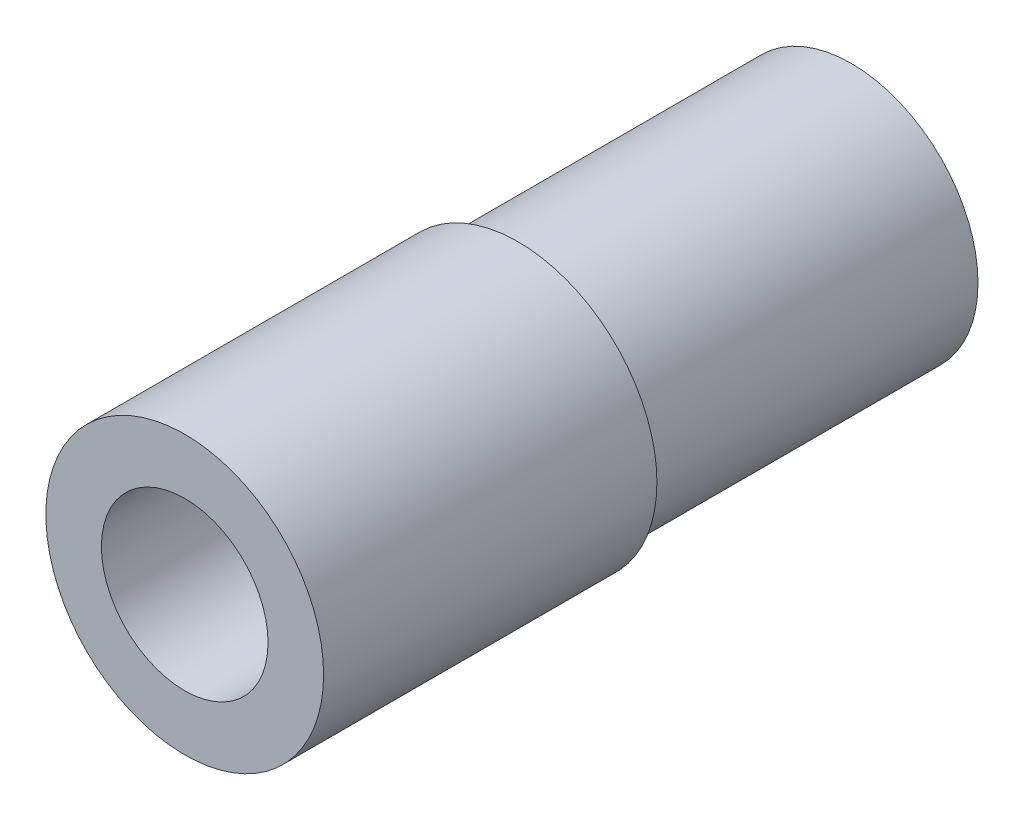
from build123d import *

# Parameters (mm, degrees)
EXTRUDE_1_DEPTH      = 20
EXTRUDE_1_DEPTH_BACK = 10
SKETCH_1_R           = 11.4
SKETCH_2_R           = 12.5
EXTRUDE_2_DEPTH      = 30


with BuildPart() as part:
    # 草图1 → 凸台-拉伸1 (new, two sides: drawn at the far end of the back side and taken through both)
    with BuildSketch(Plane.XY.offset(-EXTRUDE_1_DEPTH_BACK)):
        Circle(SKETCH_1_R)
    extrude(amount=EXTRUDE_1_DEPTH + EXTRUDE_1_DEPTH_BACK)

    # 草图2 → 凸台-拉伸2 (add)
    with BuildSketch(Plane.XY.offset(20)):
        Circle(SKETCH_2_R)
    extrude(amount=EXTRUDE_2_DEPTH)

    # 草图7 → 切除-旋转1 (revolve, cut)
    with BuildSketch(Plane(origin=(0, 0, 0), x_dir=(0, 0, -1), z_dir=(1, 0, 0)), mode=Mode.PRIVATE) as cut_revolve_1_sk:
        Polygon((-50, 0), (-18, 0), (-22.506454643, 7.5), (-50, 7.5), align=None)
    revolve(cut_revolve_1_sk.sketch.rotate(Axis((0, 0, 50), (0, 0, -1)), 90), axis=Axis((0, 0, 50), (0, 0, -1)), mode=Mode.SUBTRACT)


solid = part.part
